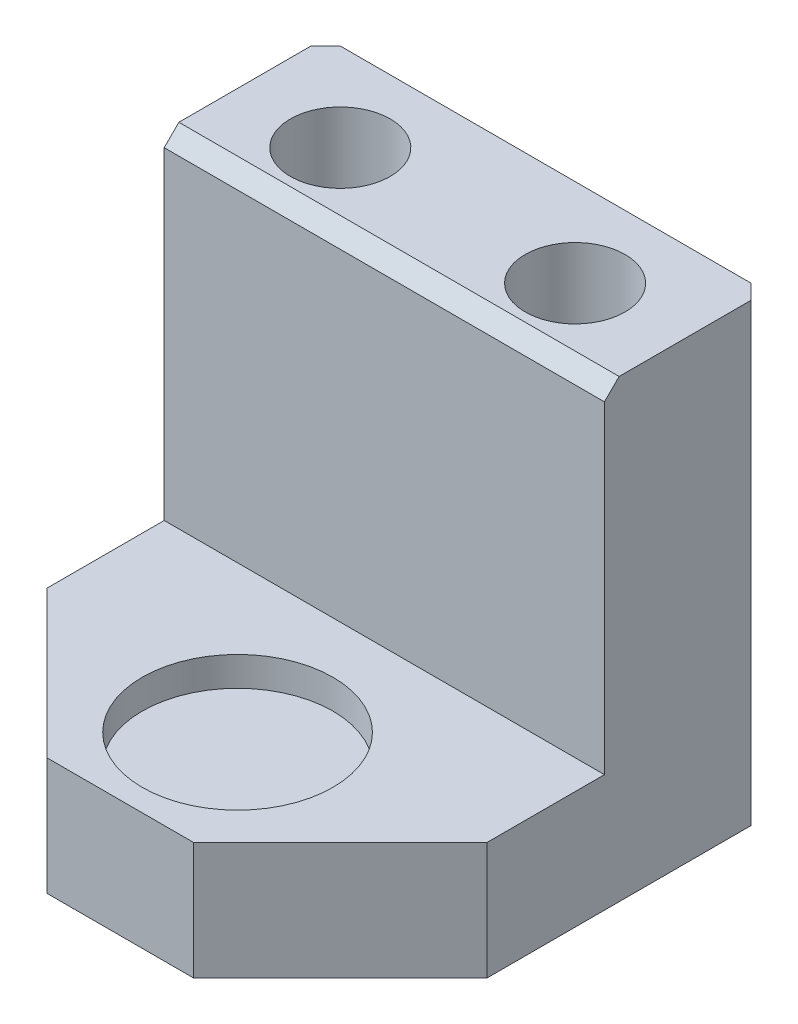
from build123d import *

# Parameters (mm, degrees)
SKETCH1_W                                            = 15
SKETCH1_H                                            = 15.5
BOSS_EXTRUDE1_DEPTH                                  = 6
SKETCH2_W                                            = 15
SKETCH2_H                                            = 4
BOSS_EXTRUDE2_DEPTH                                  = 9
SKETCH3_R                                            = 3.25
CUT_EXTRUDE1_DEPTH                                   = 1
HOLE_SIZE_PER_SOCKET_HEAD_CAP_SCREW_TYPE_D           = 3.4
HOLE_SIZE_PER_SOCKET_HEAD_CAP_SCREW_TYPE_CBORE_D     = 6
HOLE_SIZE_PER_SOCKET_HEAD_CAP_SCREW_TYPE_CBORE_DEPTH = 3.4
CHAMFER1_SIZE                                        = 5
CHAMFER2_SIZE                                        = 1
CHAMFER3_SIZE                                        = 0.5


with BuildPart() as part:
    # Sketch1 → Boss-Extrude1 (new body)
    with BuildSketch(Plane.XY):
        Rectangle(SKETCH1_W, SKETCH1_H)
    extrude(amount=BOSS_EXTRUDE1_DEPTH)

    # Sketch2 → Boss-Extrude2 (add)
    with BuildSketch(Plane.XY.offset(6)):
        with Locations((0, -5.75)):
            Rectangle(SKETCH2_W, SKETCH2_H)
    extrude(amount=BOSS_EXTRUDE2_DEPTH)

    # Sketch3 → Cut-Extrude1 (cut)
    with BuildSketch(Plane(origin=(0, -3.75, 0), x_dir=(1, 0, 0), z_dir=(0, 1, 0))):
        with Locations(Location((0, -11, 0), (0, 0, 270))):
            Circle(SKETCH3_R)
    extrude(amount=-CUT_EXTRUDE1_DEPTH, mode=Mode.SUBTRACT)

    # Hole size per socket head cap screw type 1 (through all)
    with Locations(Plane(origin=(0, -7.75, 0), x_dir=(-1, 0, 0), z_dir=(0, -1, 0))):
        with Locations((4, -3.5), (-4, -3.5)):
            CounterBoreHole(HOLE_SIZE_PER_SOCKET_HEAD_CAP_SCREW_TYPE_D / 2, HOLE_SIZE_PER_SOCKET_HEAD_CAP_SCREW_TYPE_CBORE_D / 2, HOLE_SIZE_PER_SOCKET_HEAD_CAP_SCREW_TYPE_CBORE_DEPTH)

    # Chamfer1
    chamfer1_edges = [part.edges().sort_by_distance(p)[0] for p in [
        (-7.5, -5.75, 15),
        (7.5, -5.75, 15),
    ]]
    chamfer(chamfer1_edges, length=CHAMFER1_SIZE)

    # Chamfer2
    chamfer2_edges = [part.edges().sort_by_distance(p)[0] for p in [
        (-7.5, 0, 0),
        (7.5, 0, 0),
    ]]
    chamfer(chamfer2_edges, length=CHAMFER2_SIZE)

    # Chamfer3
    chamfer3_edges = [part.edges().sort_by_distance(p)[0] for p in [
        (0, 7.75, 6),
        (0, 7.75, 0),
    ]]
    chamfer(chamfer3_edges, length=CHAMFER3_SIZE)


solid = part.part
